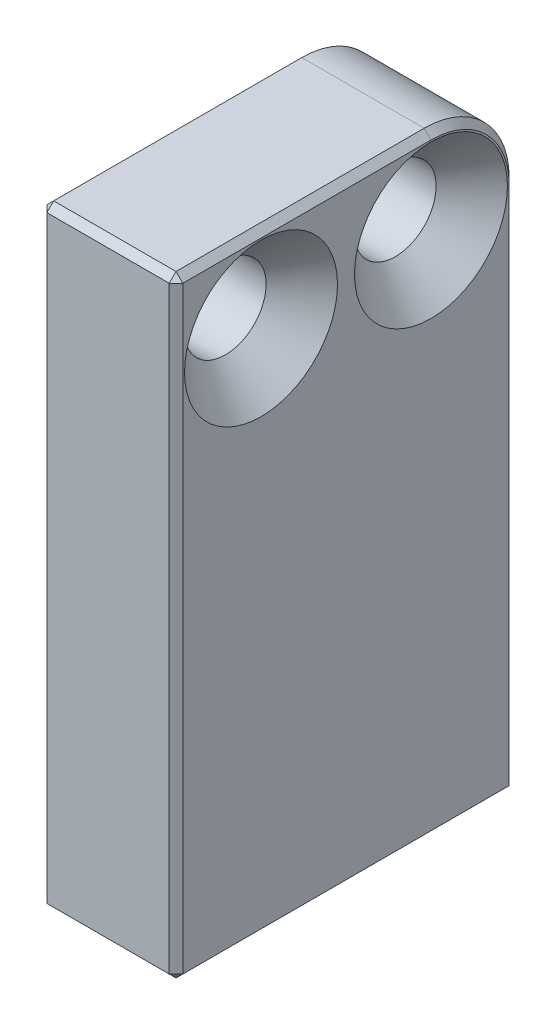
SolidWorks part; units mm, degrees
material "7075-T6"
ref_plane "Front Plane" through (0, 0, 0) normal (0, 0, 1) x (1, 0, 0)
ref_plane "Top Plane" through (0, 0, 0) normal (0, 1, 0) x (1, 0, 0)
ref_plane "Right Plane" through (0, 0, 0) normal (1, 0, 0) x (0, 0, -1)
sketch "Sketch1" plane through (0, 0, 0) normal (0, 1, 0) x (1, 0, 0)
  line L1 (0, 0) -> (4, 0)
  line L2 (0, 0) -> (0, 10)
  line L3 (0, 10) -> (4, 10)
  line L4 (4, 0) -> (4, 10)
  dimension "D1" = 10
  dimension "D2" = 4
extrude "Boss-Extrude1" add sketch "Sketch1" along normal blind 18
hole_wizard "Hole size slotted countersunk wood screw type 1" positions "Sketch2" profile "Sketch3" countersink size "M2" standard "GB" end condition up to next
sketch "Sketch2" plane through (4, 0, 0) normal (1, 0, 0) x (0, 0, -1)
  line L0 (7.5, 15.5) -> (2.5, 15.5)
  line L2 (0, 18) -> (10, 18) construction
  line L3 (10, 18) -> (10, 0) construction
  point P0 (2.5, 15.5)
  point P2 (7.5, 15.5)
  dimension "D1" = 5
  dimension "D2" = 2.5
  dimension "D3" = 2.5
sketch "Sketch3" plane through (4, 15.5, -2.5) normal (0, 1, 0) x (0, 0, -1)
  line L0 (0, 0) -> (0, 4)
  line L1 (0, 4) -> (1.2, 4)
  line L2 (1.2, 4) -> (1.2, 1.05)
  line L3 (1.2, 1.05) -> (2.25, 0)
  line L5 (2.25, 0) -> (0, 0)
  line L6 (-1.2, 1.05) -> (-2.25, 0) construction
  line L11 (0, -6.35) -> (0, 107.95) construction
  dimension "通孔孔直径" = 2.4
  dimension "通孔孔深度" = 4
  dimension "近端锥形沉头孔直径" = 4.5
  dimension "近端锥形沉头孔角度" = 90
hole_wizard "M2 Tapped Hole1" positions "Sketch4" profile "Sketch5" tap size "M2" standard "GB"
sketch "Sketch4" plane through (0, 0, 0) normal (0, -1, 0) x (-1, 0, 0)
  line L0 (-2, 2.5) -> (-2, 7.5)
  line L2 (-4, 0) -> (-4, 10) construction
  line L3 (-4, 10) -> (0, 10) construction
  point P0 (-2, 2.5)
  point P2 (-2, 7.5)
  dimension "D1" = 5
  dimension "D2" = 2
  dimension "D3" = 2.5
sketch "Sketch5" plane through (2, 0, -2.5) normal (1, 0, 0) x (0, 0, -1)
  line L0 (0, 0) -> (0, 6.8807)
  line L1 (0, 6.8807) -> (0.8, 6.4)
  line L2 (0.8, 6.4) -> (0.8, 0)
  line L5 (0.8, 0) -> (0, 0)
  line L10 (0, 6.8807) -> (-0.8, 6.4) construction
  line L11 (0, -6.35) -> (0, 107.95) construction
  dimension "螺纹孔钻头直径" = 1.6
  dimension "螺纹孔钻头深度" = 6.4
  dimension "导头角度" = 118
cosmetic thread "Cosmetic Thread1" parameters "D1"=5.2, "D2"=2
cosmetic thread "Cosmetic Thread2" parameters "D1"=5.2, "D2"=2
fillet "Fillet1" radius 2.5 1 edges at (2, 18, -10)
chamfer "Chamfer1" distance 0.2 angle 45 17 edges at (2, 0, -8.3) (2, 0, -3.3) (4, 7.75, -10) (4, 17.2678, -9.2678) (4, 0, -5) (2, 0, -10) (4, 18, -3.75) (2, 18, 0) (4, 9, 0) (2, 0, 0) (0, 9, 0) (0, 0, -5) (0, 7.75, -10) (0, 17.2678, -9.2678) (0, 18, -3.75) (0, 15.5, -8.7) (0, 15.5, -3.7)
